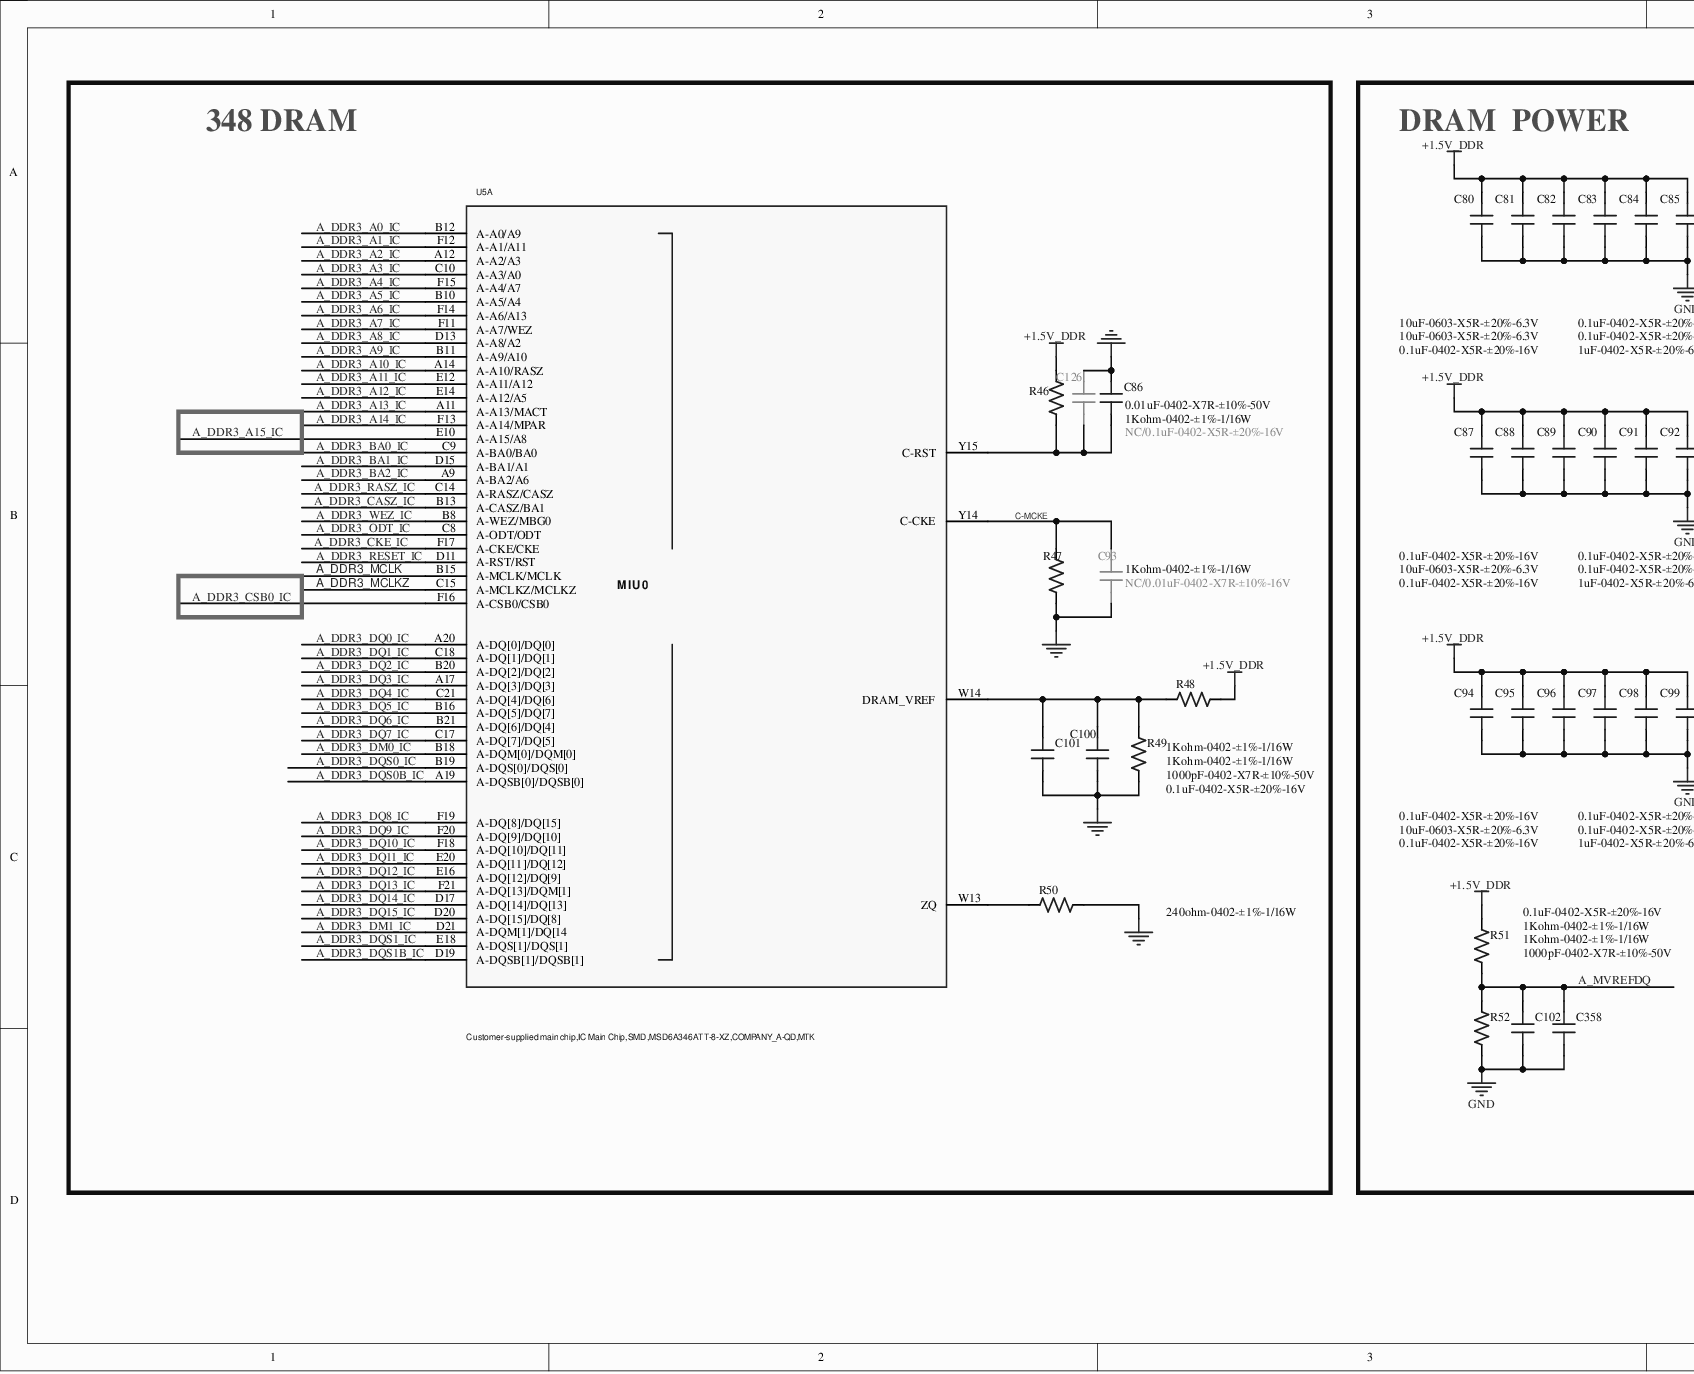
[diagram p0: MISC84395-10.SchDoc, left]
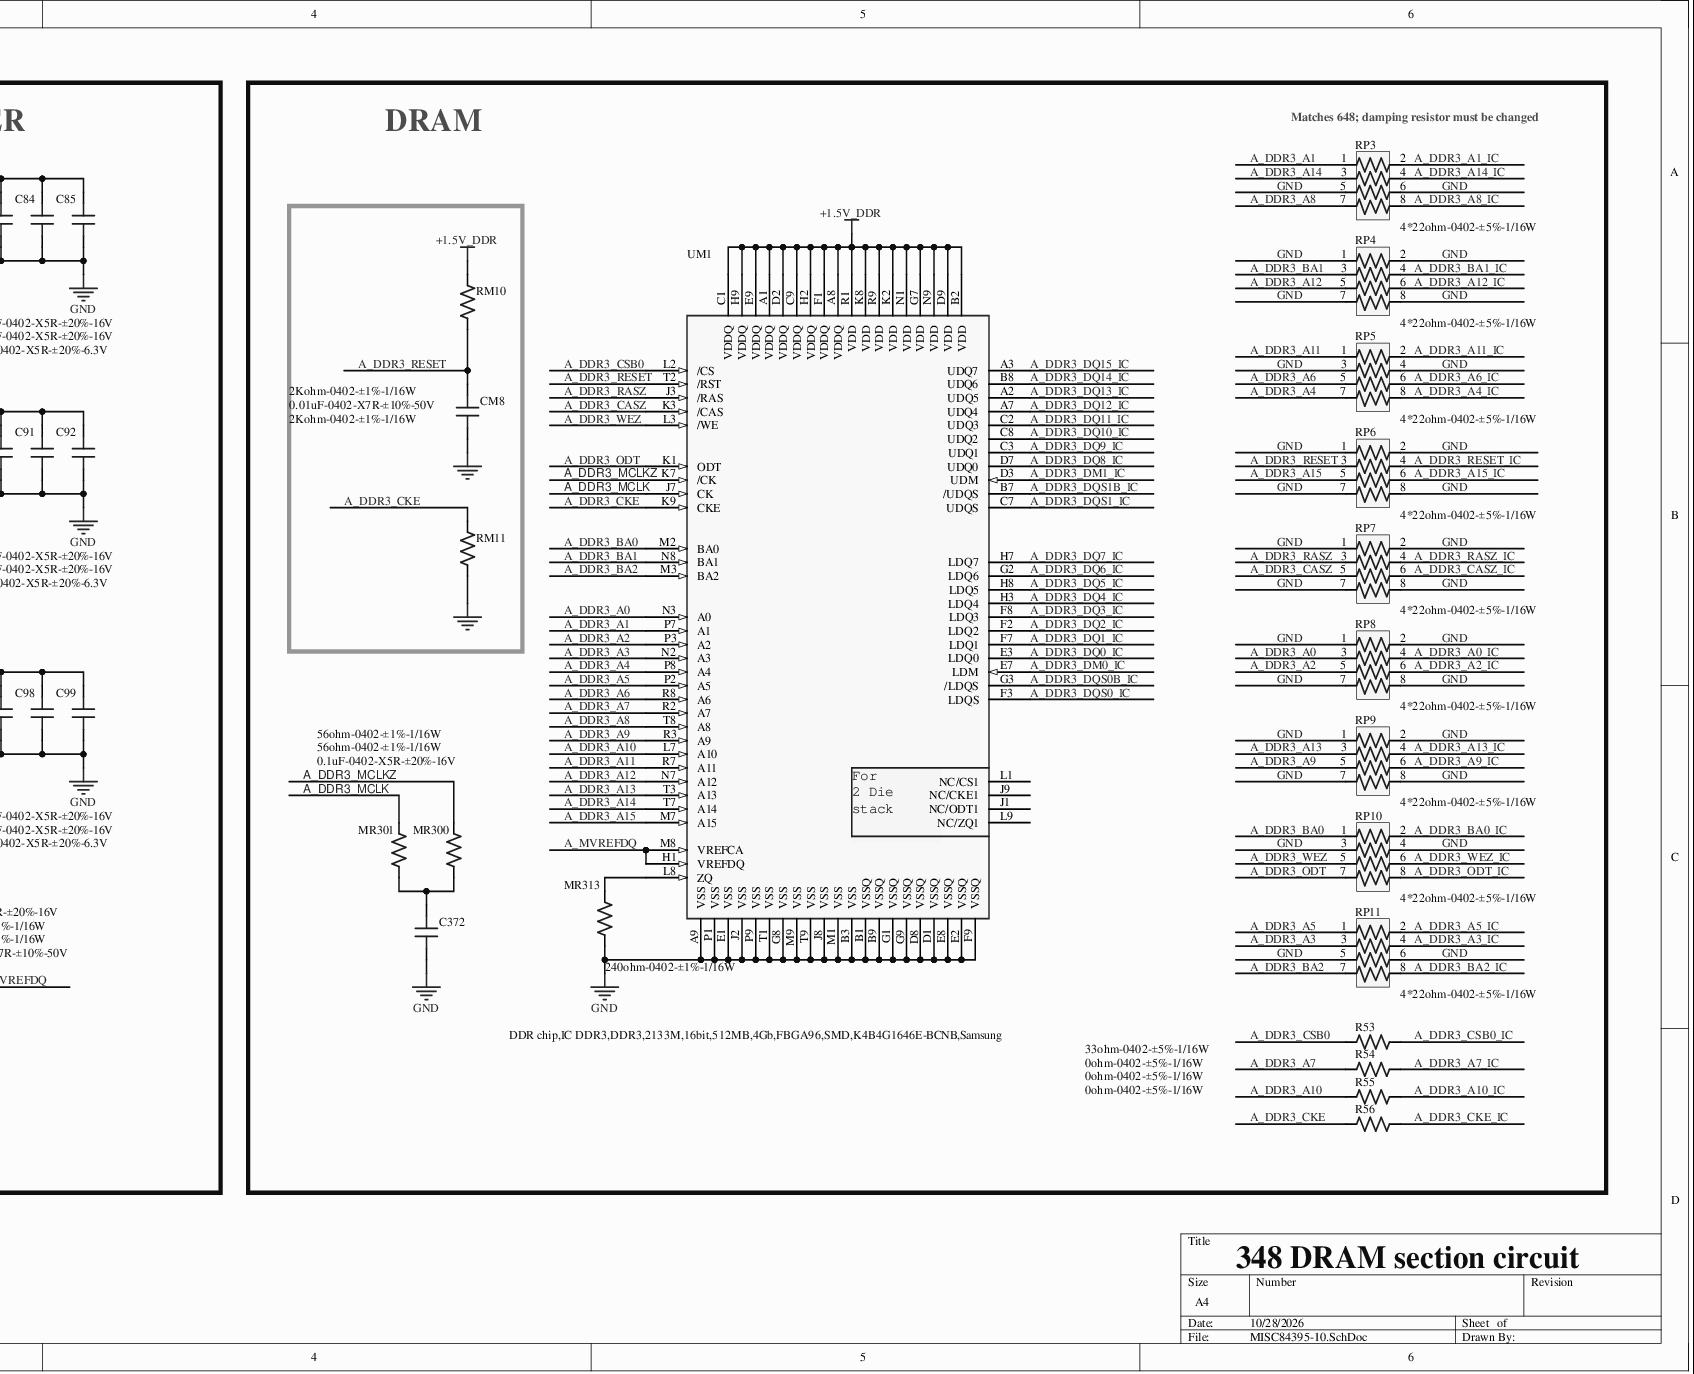
[diagram p1: MISC84395-10.SchDoc, right]
# Altium project MISC84395-37.PrjPCB (part 7 of 13)

## Sheet MISC84395-10.SchDoc
size 609 x 254 mm

### Parts
C80  10uF-0603-X5R-±20%-6.3V  [C0603]
C81  10uF-0603-X5R-±20%-6.3V  [C0603]
C82  0.1uF-0402-X5R-±20%-16V  [C0402]
C83  0.1uF-0402-X5R-±20%-16V  [C0402]
C84  0.1uF-0402-X5R-±20%-16V  [C0402]
C85  1uF-0402-X5R-±20%-6.3V  [C0402]
C86  0.01uF-0402-X7R-±10%-50V  [C0402]
C87  10uF-0603-X5R-±20%-6.3V  [C0603]
C88  0.1uF-0402-X5R-±20%-16V  [C0402]
C89  0.1uF-0402-X5R-±20%-16V  [C0402]
C90  0.1uF-0402-X5R-±20%-16V  [C0402]
C91  0.1uF-0402-X5R-±20%-16V  [C0402]
C92  1uF-0402-X5R-±20%-6.3V  [C0402]
C93  NC/0.01uF-0402-X7R-±10%-16V  [C0402]
C94  10uF-0603-X5R-±20%-6.3V  [C0603]
C95  0.1uF-0402-X5R-±20%-16V  [C0402]
C96  0.1uF-0402-X5R-±20%-16V  [C0402]
C97  0.1uF-0402-X5R-±20%-16V  [C0402]
C98  0.1uF-0402-X5R-±20%-16V  [C0402]
C99  1uF-0402-X5R-±20%-6.3V  [C0402]
C100  0.1uF-0402-X5R-±20%-16V  [C0402]
C101  1000pF-0402-X7R-±10%-50V  [C0402]
C102  1000pF-0402-X7R-±10%-50V  [C0402]
C126  NC/0.1uF-0402-X5R-±20%-16V  [C0402]
C358  0.1uF-0402-X5R-±20%-16V  [C0402]
C372  0.1uF-0402-X5R-±20%-16V  [C0402]
CM8  0.01uF-0402-X7R-±10%-50V  [C0402]
MR300  56ohm-0402-±1%-1/16W  [R0402]
MR301  56ohm-0402-±1%-1/16W  [R0402]
MR313  240ohm-0402-±1%-1/16W  [R0402]
R46  1Kohm-0402-±1%-1/16W  [R0402]
R47  1Kohm-0402-±1%-1/16W  [R0402]
R48  1Kohm-0402-±1%-1/16W  [R0402]
R49  1Kohm-0402-±1%-1/16W  [R0402]
R50  240ohm-0402-±1%-1/16W  [R0402]
R51  1Kohm-0402-±1%-1/16W  [R0402]
R52  1Kohm-0402-±1%-1/16W  [R0402]
R53  33ohm-0402-±5%-1/16W  [R0402]
R54  0ohm-0402-±5%-1/16W  [R0402]
R55  0ohm-0402-±5%-1/16W  [R0402]
R56  0ohm-0402-±5%-1/16W  [R0402]
RM10  2Kohm-0402-±1%-1/16W  [R0402]
RM11  2Kohm-0402-±1%-1/16W  [R0402]
RP3  4*22ohm-0402-±5%-1/16W  [RA0402]
RP4  4*22ohm-0402-±5%-1/16W  [RA0402]
RP5  4*22ohm-0402-±5%-1/16W  [RA0402]
RP6  4*22ohm-0402-±5%-1/16W  [RA0402]
RP7  4*22ohm-0402-±5%-1/16W  [RA0402]
RP8  4*22ohm-0402-±5%-1/16W  [RA0402]
RP9  4*22ohm-0402-±5%-1/16W  [RA0402]
RP10  4*22ohm-0402-±5%-1/16W  [RA0402]
RP11  4*22ohm-0402-±5%-1/16W  [RA0402]
U5  Customer-supplied main chip,IC Main Chip,SMD,MSD6A346ATT-8-XZ,COMPANY_A-QD,MTK  [BGA406/0.8]  (part A of 7)
UM1  DDR chip,IC DDR3,DDR3,2133M,16bit,512MB,4Gb,FBGA96,SMD,K4B4G1646E-BCNB,Samsung  [BGA96/0.8-1]

### Blocks framed on the sheet
348 DRAM: C86 C93 C100 C101 C126 R46-R50 U5
DRAM  POWER: C80-C85 C87-C92 C94-C99 C102 C358 R51 R52
DRAM: C372 CM8 MR300 MR301 MR313 R53-R56 RM10 RM11 RP3-RP11 UM1

### Nets
+1.5V_DDR: C80.2 C81.2 C82.2 C83.2 C84.2 C85.2 C87.2 C88.2 C89.2 C90.2 C91.2 C92.2 C94.2 C95.2 C96.2 C97.2 C98.2 C99.2 R46.2 R48.1 R51.2 RM10.2 UM1.A1(VDDQ) UM1.A8(VDDQ) UM1.B2(VDD) UM1.C1(VDDQ) UM1.C9(VDDQ) UM1.D2(VDDQ) UM1.D9(VDD) UM1.E9(VDDQ) UM1.F1(VDDQ) UM1.G7(VDD) UM1.H2(VDDQ) UM1.H9(VDDQ) UM1.K2(VDD) UM1.K8(VDD) UM1.N1(VDD) UM1.N9(VDD) UM1.R1(VDD) UM1.R9(VDD)
GND: C80.1 C81.1 C82.1 C83.1 C84.1 C85.1 C86.2 C87.1 C88.1 C89.1 C90.1 C91.1 C92.1 C93.1 C94.1 C95.1 C96.1 C97.1 C98.1 C99.1 C100.1 C101.2 C102.2 C126.2 C358.1 C372.1 CM8.1 MR313.1 R47.1 R49.2 R50.2 R52.1 RM11.1 RP3.5 RP3.6 RP4.1 RP4.2 RP4.7 RP4.8 RP5.3 RP5.4 RP6.1 RP6.2 RP6.7 RP6.8 RP7.1 RP7.2 RP7.7 RP7.8 RP8.1 RP8.2 RP8.7 RP8.8 RP9.1 RP9.2 RP9.7 RP9.8 RP10.3 RP10.4 RP11.5 RP11.6 UM1.A9(VSS) UM1.B1(VSSQ) UM1.B3(VSS) UM1.B9(VSSQ) UM1.D1(VSSQ) UM1.D8(VSSQ) UM1.E1(VSS) UM1.E2(VSSQ) UM1.E8(VSSQ) UM1.F9(VSSQ) UM1.G1(VSSQ) UM1.G8(VSS) UM1.G9(VSSQ) UM1.J2(VSS) UM1.J8(VSS) UM1.M1(VSS) UM1.M9(VSS) UM1.P1(VSS) UM1.P9(VSS) UM1.T1(VSS) UM1.T9(VSS)
A_DDR3_A0: RP8.3 UM1.N3(A0)
A_DDR3_A0_IC: RP8.4 U5.B12(A-A0/A9)
A_DDR3_A1: RP3.1 UM1.P7(A1)
A_DDR3_A1_IC: RP3.2 U5.F12(A-A1/A11)
A_DDR3_A2: RP8.5 UM1.P3(A2)
A_DDR3_A2_IC: RP8.6 U5.A12(A-A2/A3)
A_DDR3_A3: RP11.3 UM1.N2(A3)
A_DDR3_A3_IC: RP11.4 U5.C10(A-A3/A0)
A_DDR3_A4: RP5.7 UM1.P8(A4)
A_DDR3_A4_IC: RP5.8 U5.F15(A-A4/A7)
A_DDR3_A5: RP11.1 UM1.P2(A5)
A_DDR3_A5_IC: RP11.2 U5.B10(A-A5/A4)
A_DDR3_A6: RP5.5 UM1.R8(A6)
A_DDR3_A6_IC: RP5.6 U5.F14(A-A6/A13)
A_DDR3_A7: R54.1 UM1.R2(A7)
A_DDR3_A7_IC: R54.2 U5.F11(A-A7/WEZ)
A_DDR3_A8: RP3.7 UM1.T8(A8)
A_DDR3_A8_IC: RP3.8 U5.D13(A-A8/A2)
A_DDR3_A9: RP9.5 UM1.R3(A9)
A_DDR3_A9_IC: RP9.6 U5.B11(A-A9/A10)
A_DDR3_A10: R55.1 UM1.L7(A10)
A_DDR3_A10_IC: R55.2 U5.A14(A-A10/RASZ)
A_DDR3_A11: RP5.1 UM1.R7(A11)
A_DDR3_A11_IC: RP5.2 U5.E12(A-A11/A12)
A_DDR3_A12: RP4.5 UM1.N7(A12)
A_DDR3_A12_IC: RP4.6 U5.E14(A-A12/A5)
A_DDR3_A13: RP9.3 UM1.T3(A13)
A_DDR3_A13_IC: RP9.4 U5.A11(A-A13/MACT)
A_DDR3_A14: RP3.3 UM1.T7(A14)
A_DDR3_A14_IC: RP3.4 U5.F13(A-A14/MPAR)
A_DDR3_A15: RP6.5 UM1.M7(A15)
A_DDR3_A15_IC: RP6.6 U5.E10(A-A15/A8)
A_DDR3_BA0: RP10.1 UM1.M2(BA0)
A_DDR3_BA0_IC: RP10.2 U5.C9(A-BA0/BA0)
A_DDR3_BA1: RP4.3 UM1.N8(BA1)
A_DDR3_BA1_IC: RP4.4 U5.D15(A-BA1/A1)
A_DDR3_BA2: RP11.7 UM1.M3(BA2)
A_DDR3_BA2_IC: RP11.8 U5.A9(A-BA2/A6)
A_DDR3_CASZ: RP7.5 UM1.K3(/CAS)
A_DDR3_CASZ_IC: RP7.6 U5.B13(A-CASZ/BA1)
A_DDR3_CKE: R56.1 RM11.2 UM1.K9(CKE)
A_DDR3_CKE_IC: R56.2 U5.F17(A-CKE/CKE)
A_DDR3_CSB0: R53.1 UM1.L2(/CS)
A_DDR3_CSB0_IC: R53.2 U5.F16(A-CSB0/CSB0)
A_DDR3_DM0_IC: U5.B18(A-DQM[0]/DQM[0]) UM1.E7(LDM)
A_DDR3_DM1_IC: U5.D21(A-DQM[1]/DQ[14) UM1.D3(UDM)
A_DDR3_DQ0_IC: U5.A20(A-DQ[0]/DQ[0]) UM1.E3(LDQ0)
A_DDR3_DQ1_IC: U5.C18(A-DQ[1]/DQ[1]) UM1.F7(LDQ1)
A_DDR3_DQ2_IC: U5.B20(A-DQ[2]/DQ[2]) UM1.F2(LDQ2)
A_DDR3_DQ3_IC: U5.A17(A-DQ[3]/DQ[3]) UM1.F8(LDQ3)
A_DDR3_DQ4_IC: U5.C21(A-DQ[4]/DQ[6]) UM1.H3(LDQ4)
A_DDR3_DQ5_IC: U5.B16(A-DQ[5]/DQ[7]) UM1.H8(LDQ5)
A_DDR3_DQ6_IC: U5.B21(A-DQ[6]/DQ[4]) UM1.G2(LDQ6)
A_DDR3_DQ7_IC: U5.C17(A-DQ[7]/DQ[5]) UM1.H7(LDQ7)
A_DDR3_DQ8_IC: U5.F19(A-DQ[8]/DQ[15]) UM1.D7(UDQ0)
A_DDR3_DQ9_IC: U5.F20(A-DQ[9]/DQ[10]) UM1.C3(UDQ1)
A_DDR3_DQ10_IC: U5.F18(A-DQ[10]/DQ[11]) UM1.C8(UDQ2)
A_DDR3_DQ11_IC: U5.E20(A-DQ[11]/DQ[12]) UM1.C2(UDQ3)
A_DDR3_DQ12_IC: U5.E16(A-DQ[12]/DQ[9]) UM1.A7(UDQ4)
A_DDR3_DQ13_IC: U5.F21(A-DQ[13]/DQM[1]) UM1.A2(UDQ5)
A_DDR3_DQ14_IC: U5.D17(A-DQ[14]/DQ[13]) UM1.B8(UDQ6)
A_DDR3_DQ15_IC: U5.D20(A-DQ[15]/DQ[8]) UM1.A3(UDQ7)
A_DDR3_DQS0_IC: U5.B19(A-DQS[0]/DQS[0]) UM1.F3(LDQS)
A_DDR3_DQS0B_IC: U5.A19(A-DQSB[0]/DQSB[0]) UM1.G3(/LDQS)
A_DDR3_DQS1_IC: U5.E18(A-DQS[1]/DQS[1]) UM1.C7(UDQS)
A_DDR3_DQS1B_IC: U5.D19(A-DQSB[1]/DQSB[1]) UM1.B7(/UDQS)
A_DDR3_MCLK: MR301.2 U5.B15(A-MCLK/MCLK) UM1.J7(CK)
A_DDR3_MCLKZ: MR300.2 U5.C15(A-MCLKZ/MCLKZ) UM1.K7(/CK)
A_DDR3_ODT: RP10.7 UM1.K1(ODT)
A_DDR3_ODT_IC: RP10.8 U5.C8(A-ODT/ODT)
A_DDR3_RASZ: RP7.3 UM1.J3(/RAS)
A_DDR3_RASZ_IC: RP7.4 U5.C14(A-RASZ/CASZ)
A_DDR3_RESET: CM8.2 RM10.1 RP6.3 UM1.T2(/RST)
A_DDR3_RESET_IC: RP6.4 U5.D11(A-RST/RST)
A_DDR3_WEZ: RP10.5 UM1.L3(/WE)
A_DDR3_WEZ_IC: RP10.6 U5.B8(A-WEZ/MBG0)
A_MVREFDQ: C102.1 C358.2 R51.1 R52.2 UM1.H1(VREFDQ) UM1.M8(VREFCA)
C-MCKE: C93.2 R47.2 U5.Y14(C-CKE)
NetC86_1: C86.1 C126.1 R46.1 U5.Y15(C-RST)
NetC100_2: C100.2 C101.1 R48.2 R49.1 U5.W14(DRAM_VREF)
NetC372_2: C372.2 MR300.1 MR301.1
NetMR313_2: MR313.2 UM1.L8(ZQ)
NetR50_1: R50.1 U5.W13(ZQ)

Not connected (* = marked no-connect by the designer): UM1 J1(NC/ODT1)* J9(NC/CKE1)* L1(NC/CS1)* L9(NC/ZQ1)*

### Notes on the sheet
- (near RP3) Matches 648; damping resistor must be changed
- 348 DRAM section circuit

### Library data of the parts
C80 C81 C87 C94 = 10uF-0603-X5R-±20%-6.3V-D
C82-C84 C88-C91 C95-C98 C100 C126 C358 = 0.1uF-0402-X7R-±10%-16V-D
C85 C92 C99 = 1uF-0402-X5R-±20%-6.3V-D
C86 CM8 = 0.01uF-0402-X7R-±10%-50V-D
C93 = 0.01uF-0402-X7R-±10%-16V-D
C101 C102 = 1000pF-0402-X7R-±10%-50V-D
C372 = 0.1uF-0402-X5R-±20%-16V-D
MR300 MR301 = 56ohm-0402-±5%-1/16W-D
MR313 R50 = 240ohm-0402-±1%-1/16W-D
R46-R49 R51 R52 = 1Kohm-0402-±1%-1/16W-D
R53-R56 = 0ohm-0402-±5%-1/16W-D
RM10 RM11 = 2Kohm-0402-±1%-1/16W-D
RP3-RP11 = 4*0ohm-0402-±5%-1/16W-D
U5 = 004.016.0000830: TV main chip,IC Main Chip,MSD6A348AT-X1,CAN TV,32bit,Multi-Core,BGA406,SMD,Mstar-D
UM1 = NT5CB256M16CP-DI-D

## Sheet MISC84395-11.SchDoc
size 243 x 165 mm
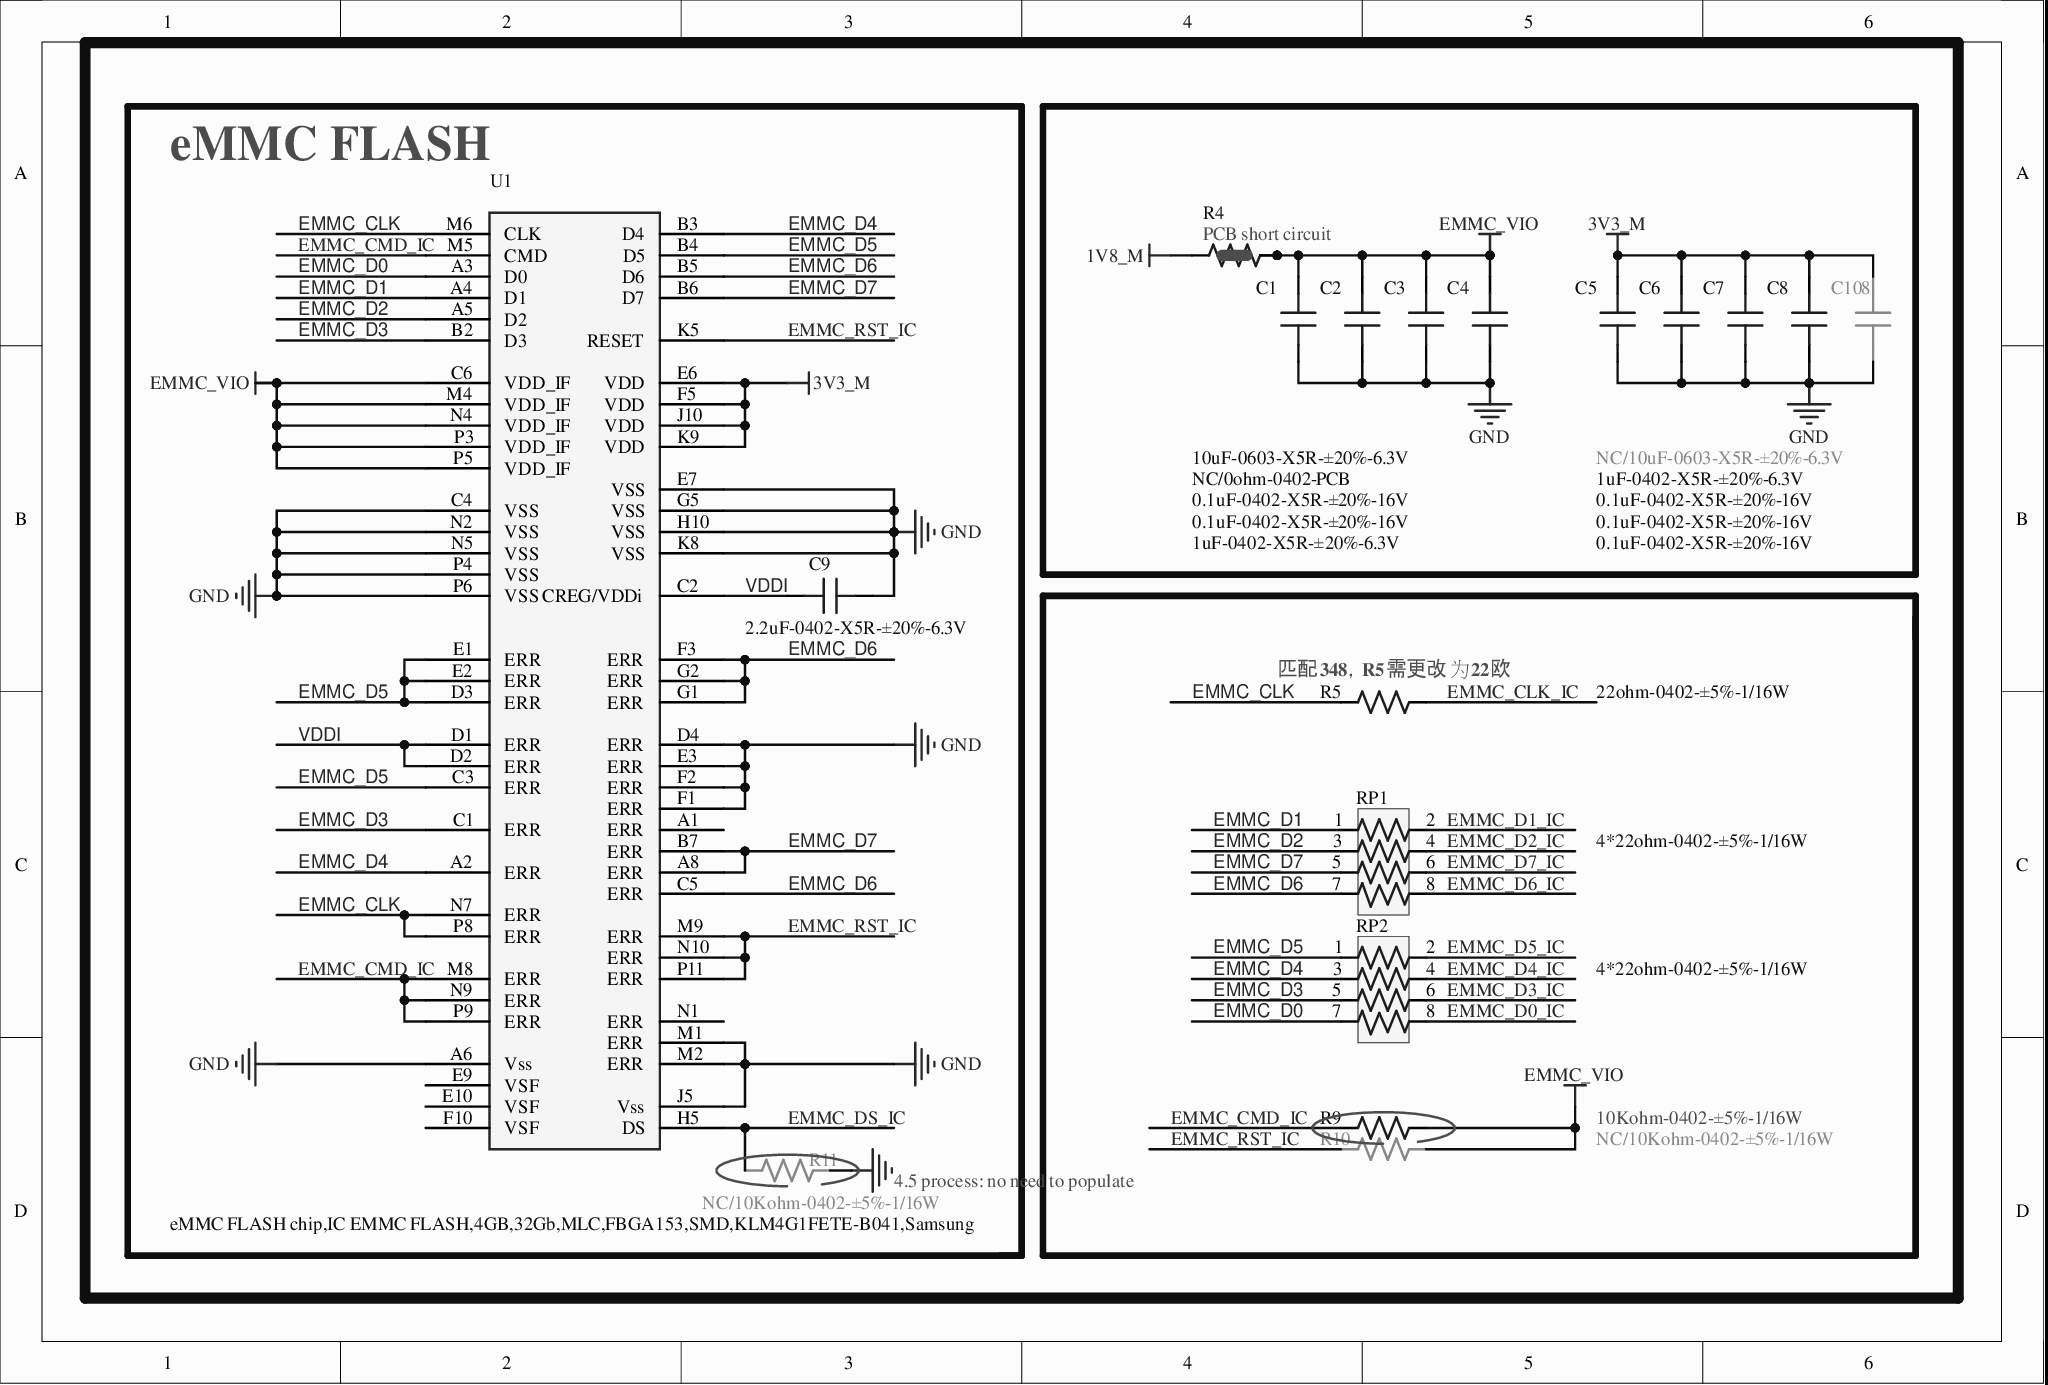
[diagram p2: MISC84395-11.SchDoc]

### Parts
C1  10uF-0603-X5R-±20%-6.3V  [C0603]
C2  1uF-0402-X5R-±20%-6.3V  [C0402]
C3  0.1uF-0402-X5R-±20%-16V  [C0402]
C4  0.1uF-0402-X5R-±20%-16V  [C0402]
C5  1uF-0402-X5R-±20%-6.3V  [C0402]
C6  0.1uF-0402-X5R-±20%-16V  [C0402]
C7  0.1uF-0402-X5R-±20%-16V  [C0402]
C8  0.1uF-0402-X5R-±20%-16V  [C0402]
C9  2.2uF-0402-X5R-±20%-6.3V  [C0402]
C108  NC/10uF-0603-X5R-±20%-6.3V  [C0603]
R4  NC/0ohm-0402-PCB  [R0402SC]
R5  22ohm-0402-±5%-1/16W  [R0402]
R9  10Kohm-0402-±5%-1/16W  [R0402]
R10  NC/10Kohm-0402-±5%-1/16W  [R0402]
R11  NC/10Kohm-0402-±5%-1/16W  [R0402]
RP1  4*22ohm-0402-±5%-1/16W  [RA0402]
RP2  4*22ohm-0402-±5%-1/16W  [RA0402]
U1  eMMC FLASH chip,IC EMMC FLASH,4GB,32Gb,MLC,FBGA153,SMD,KLM4G1FETE-B041,Samsung  [BGA153/0.5-1]

### Nets
1V8_M: R4.1
3V3_M: C5.2 C6.2 C7.2 C8.2 C108.2 U1.E6(VDD) U1.F5(VDD) U1.J10(VDD) U1.K9(VDD)
EMMC_VIO: C1.2 C2.2 C3.2 C4.2 R4.2 R4.3 R9.2 R10.2 U1.C6(VDD_IF) U1.M4(VDD_IF) U1.N4(VDD_IF) U1.P3(VDD_IF) U1.P5(VDD_IF)
GND: C1.1 C2.1 C3.1 C4.1 C5.1 C6.1 C7.1 C8.1 C9.2 C108.1 R11.1 U1.A6(Vss) U1.C4(VSS) U1.D4(ERR) U1.E3(ERR) U1.E7(VSS) U1.F1(ERR) U1.F2(ERR) U1.G5(VSS) U1.H10(VSS) U1.J5(Vss) U1.K8(VSS) U1.M1(ERR) U1.M2(ERR) U1.N2(VSS) U1.N5(VSS) U1.P4(VSS) U1.P6(VSS)
EMMC_CLK: R5.1 U1.M6(CLK) U1.N7(ERR) U1.P8(ERR)
EMMC_CLK_IC: R5.2
EMMC_CMD_IC: R9.1 U1.M5(CMD) U1.M8(ERR) U1.N9(ERR) U1.P9(ERR)
EMMC_D0: RP2.7 U1.A3(D0)
EMMC_D0_IC: RP2.8
EMMC_D1: RP1.1 U1.A4(D1)
EMMC_D1_IC: RP1.2
EMMC_D2: RP1.3 U1.A5(D2)
EMMC_D2_IC: RP1.4
EMMC_D3: RP2.5 U1.B2(D3) U1.C1(ERR)
EMMC_D3_IC: RP2.6
EMMC_D4: RP2.3 U1.A2(ERR) U1.B3(D4)
EMMC_D4_IC: RP2.4
EMMC_D5: RP2.1 U1.B4(D5) U1.C3(ERR) U1.D3(ERR) U1.E1(ERR) U1.E2(ERR)
EMMC_D5_IC: RP2.2
EMMC_D6: RP1.7 U1.B5(D6) U1.C5(ERR) U1.F3(ERR) U1.G1(ERR) U1.G2(ERR)
EMMC_D6_IC: RP1.8
EMMC_D7: RP1.5 U1.A8(ERR) U1.B6(D7) U1.B7(ERR)
EMMC_D7_IC: RP1.6
EMMC_DS_IC: R11.2 U1.H5(DS)
EMMC_RST_IC: R10.1 U1.K5(RESET) U1.M9(ERR) U1.N10(ERR) U1.P11(ERR)
VDDI: C9.1 U1.C2(CREG/VDDi) U1.D1(ERR) U1.D2(ERR)

Not connected (* = marked no-connect by the designer): U1 A1(ERR)* E9(VSF)* E10(VSF)* F10(VSF)* N1(ERR)*

### Notes on the sheet
- eMMC FLASH
- (near R5) 匹配348，R5需更改为22欧
- (near R11) 4.5 process: no need to populate

### Library data of the parts
C1 C108 = 10uF-0603-X5R-±20%-6.3V-D
C2 C5 = 1uF-0402-X5R-±20%-6.3V-D
C3 C4 C6-C8 = 0.1uF-0402-X5R-±20%-16V-D
C9 = 2.2uF-0402-X5R-±20%-6.3V-D
R4 = 0ohm-0402-PCB-D
R5 = 0ohm-0402-±5%-1/16W-D
R9 R10 = 10Kohm-0402-±5%-1/16W-D
R11 = 22ohm-0402-±5%-1/16W-D
RP1 RP2 = 4*22ohm-0402-±5%-1/16W-D
U1 = THGBMBG6D1KBAIL-D